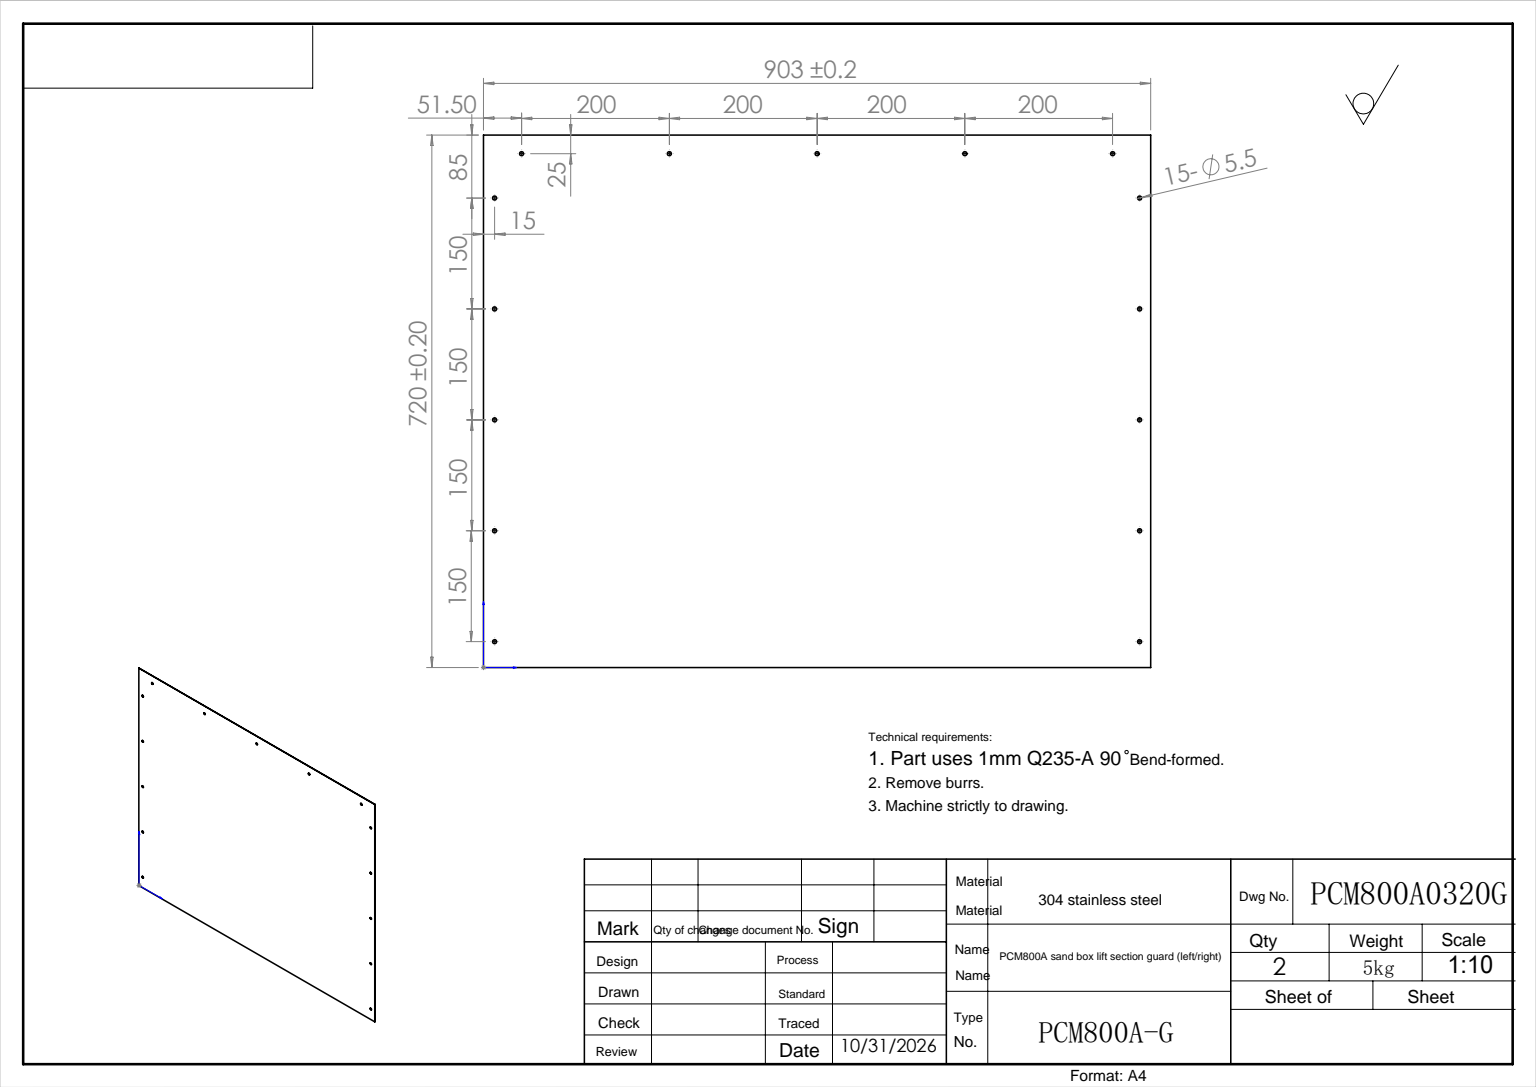
from build123d import *

# Parameters (mm, degrees)
SKETCH_1_W          = 903
SKETCH_1_H          = 720
EXTRUDE_1_DEPTH     = 1
SKETCH_2_R          = 2.75
CUT_EXTRUDE_1_DEPTH = 1.5


with BuildPart() as part:
    # 草图1 → 凸台-拉伸1 (new body)
    with BuildSketch(Plane.XY):
        with Locations((451.5, 360)):
            Rectangle(SKETCH_1_W, SKETCH_1_H)
    extrude(amount=EXTRUDE_1_DEPTH)

    # 草图2 → 切除-拉伸1 (cut)
    with BuildSketch(Plane.XY.offset(1)):
        with Locations((51.5, 695)):
            Circle(SKETCH_2_R)
        with Locations((15, 635)):
            Circle(SKETCH_2_R)
        with Locations((251.5, 695)):
            Circle(SKETCH_2_R)
        with Locations((451.5, 695)):
            Circle(SKETCH_2_R)
        with Locations((651.5, 695)):
            Circle(SKETCH_2_R)
        with Locations((851.5, 695)):
            Circle(SKETCH_2_R)
        with Locations((15, 485)):
            Circle(SKETCH_2_R)
        with Locations((15, 335)):
            Circle(SKETCH_2_R)
        with Locations((15, 185)):
            Circle(SKETCH_2_R)
        with Locations((15, 35)):
            Circle(SKETCH_2_R)
        with Locations(Location((888, 35, 0), (0, 0, 180))):
            Circle(SKETCH_2_R)
        with Locations(Location((888, 185, 0), (0, 0, 180))):
            Circle(SKETCH_2_R)
        with Locations(Location((888, 335, 0), (0, 0, 180))):
            Circle(SKETCH_2_R)
        with Locations(Location((888, 485, 0), (0, 0, 180))):
            Circle(SKETCH_2_R)
        with Locations(Location((888, 635, 0), (0, 0, 180))):
            Circle(SKETCH_2_R)
    extrude(amount=-CUT_EXTRUDE_1_DEPTH, mode=Mode.SUBTRACT)


solid = part.part
